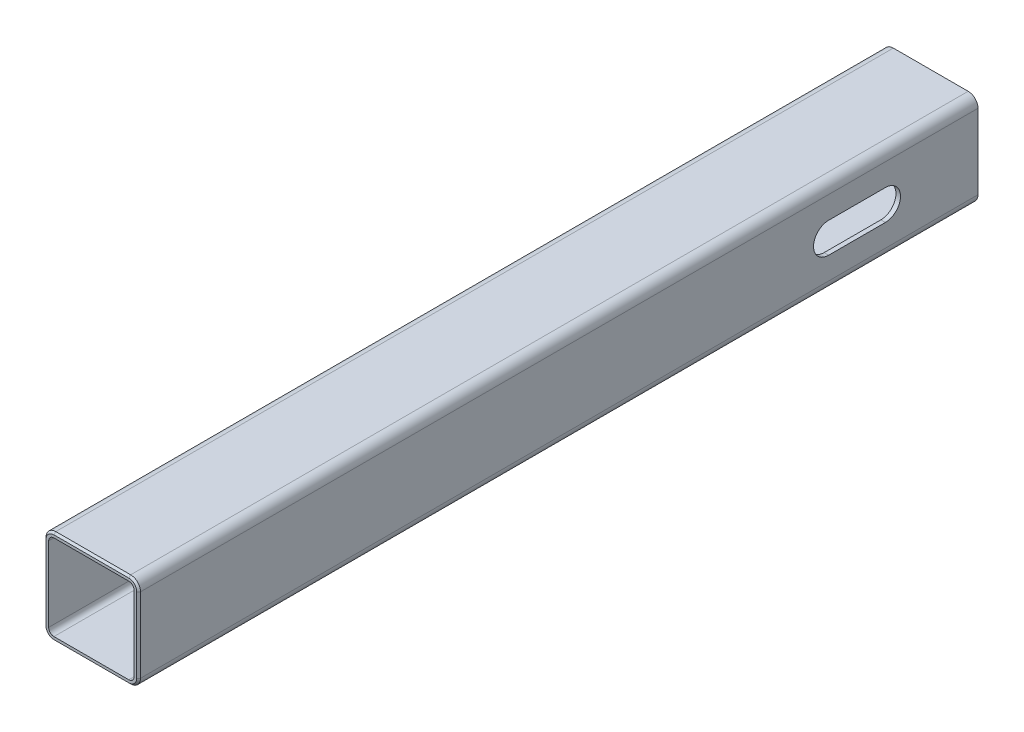
from build123d import *

# Parameters (mm, degrees)
EXTRUDE_1_DEPTH     = 2220
CHAMFER_1_SIZE      = 5
CUT_EXTRUDE_1_REACH = 2239.527


with BuildPart() as part:
    # 草图1 → 凸台-拉伸1 (new body)
    with BuildSketch(Plane.XY):
        with BuildLine():
            Line((-99, 125), (99, 125))
            ThreePointArc((99, 125), (117.384776311, 117.384776311), (125, 99))
            Line((125, 99), (125, -99))
            ThreePointArc((125, -99), (117.384776311, -117.384776311), (99, -125))
            Line((99, -125), (-99, -125))
            ThreePointArc((-99, -125), (-117.384776311, -117.384776311), (-125, -99))
            Line((-125, -99), (-125, 99))
            ThreePointArc((-125, 99), (-117.384776311, 117.384776311), (-99, 125))
        make_face()
        with BuildLine():
            Line((-99, 113), (99, 113))
            ThreePointArc((99, 113), (108.899494937, 108.899494937), (113, 99))
            Line((113, 99), (113, -99))
            ThreePointArc((113, -99), (108.899494937, -108.899494937), (99, -113))
            Line((99, -113), (-99, -113))
            ThreePointArc((-99, -113), (-108.899494937, -108.899494937), (-113, -99))
            Line((-113, -99), (-113, 99))
            ThreePointArc((-113, 99), (-108.899494937, 108.899494937), (-99, 113))
        make_face(mode=Mode.SUBTRACT)
    extrude(amount=EXTRUDE_1_DEPTH)

    # 倒角1
    chamfer_1_edges = [part.edges().sort_by_distance(p)[0] for p in [
        (-117.384776311, -117.384776311, 2220),
        (0, -125, 2220),
        (117.384776311, -117.384776311, 2220),
        (125, 0, 2220),
        (117.384776311, 117.384776311, 2220),
        (0, 125, 2220),
        (-117.384776311, 117.384776311, 2220),
        (-125, 0, 2220),
    ]]
    chamfer(chamfer_1_edges, length=CHAMFER_1_SIZE)

    # 草图2 → 切除-拉伸1 (cut, up to next)
    with BuildSketch(Plane(origin=(125, 0, 0), x_dir=(0, 0, -1), z_dir=(1, 0, 0)), mode=Mode.PRIVATE) as cut_extrude_1_sk1:
        with BuildLine():
            Line((-395, 40), (-245, 40))
            ThreePointArc((-245, 40), (-205, 0), (-245, -40))
            Line((-245, -40), (-395, -40))
            ThreePointArc((-395, -40), (-435, 0), (-395, 40))
        make_face()
    cut_extrude_1_tool1 = extrude(cut_extrude_1_sk1.sketch, amount=-CUT_EXTRUDE_1_REACH, mode=Mode.PRIVATE) & part.part
    add(cut_extrude_1_tool1.solids().sort_by_distance((125, 0, 320))[0], mode=Mode.SUBTRACT)


solid = part.part
